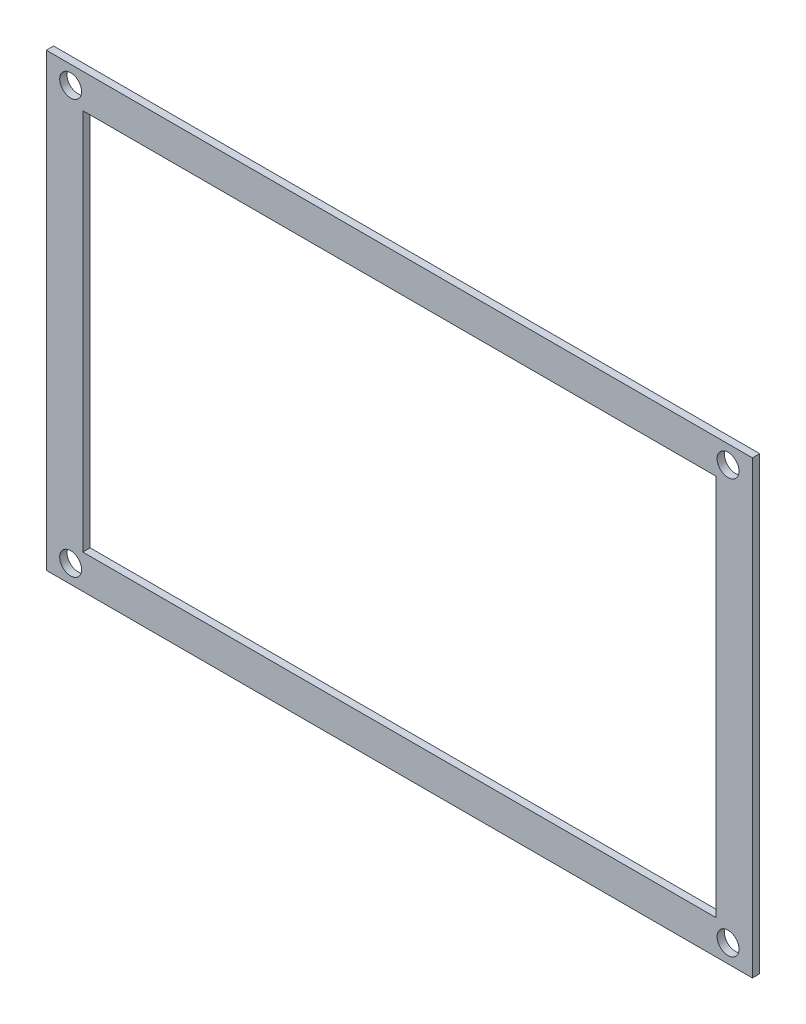
from build123d import *

# Parameters (mm, degrees)
SKETCH1_W            = 290
SKETCH1_H            = 185
SKETCH1_W_2          = 260
SKETCH1_H_2          = 157
BOSS_EXTRUDE1_DEPTH  = 3
SKETCH2_R            = 4.5
CUT_EXTRUDE1_DEPTH   = 3
LPATTERN1_COUNT      = 2
LPATTERN1_PITCH      = 270
LPATTERN1_COUNT_DIR2 = 2
LPATTERN1_PITCH_DIR2 = 170


with BuildPart() as part:
    # Sketch1 → Boss-Extrude1 (new body)
    with BuildSketch(Plane.XY):
        Rectangle(SKETCH1_W, SKETCH1_H)
        Rectangle(SKETCH1_W_2, SKETCH1_H_2, mode=Mode.SUBTRACT)
    extrude(amount=BOSS_EXTRUDE1_DEPTH)

    # Sketch2 → Cut-Extrude1 (cut)
    with BuildSketch(Plane.XY.offset(3)):
        with Locations((-135, 85)):
            Circle(SKETCH2_R)
    cut_extrude1 = extrude(amount=-CUT_EXTRUDE1_DEPTH, mode=Mode.SUBTRACT)

    # LPattern1: Cut-Extrude1 2 × 2
    with Locations(*[(i * LPATTERN1_PITCH, -j * LPATTERN1_PITCH_DIR2, 0) for i in range(LPATTERN1_COUNT) for j in range(LPATTERN1_COUNT_DIR2) if (i, j) != (0, 0)]):
        add(cut_extrude1, mode=Mode.SUBTRACT)


solid = part.part
